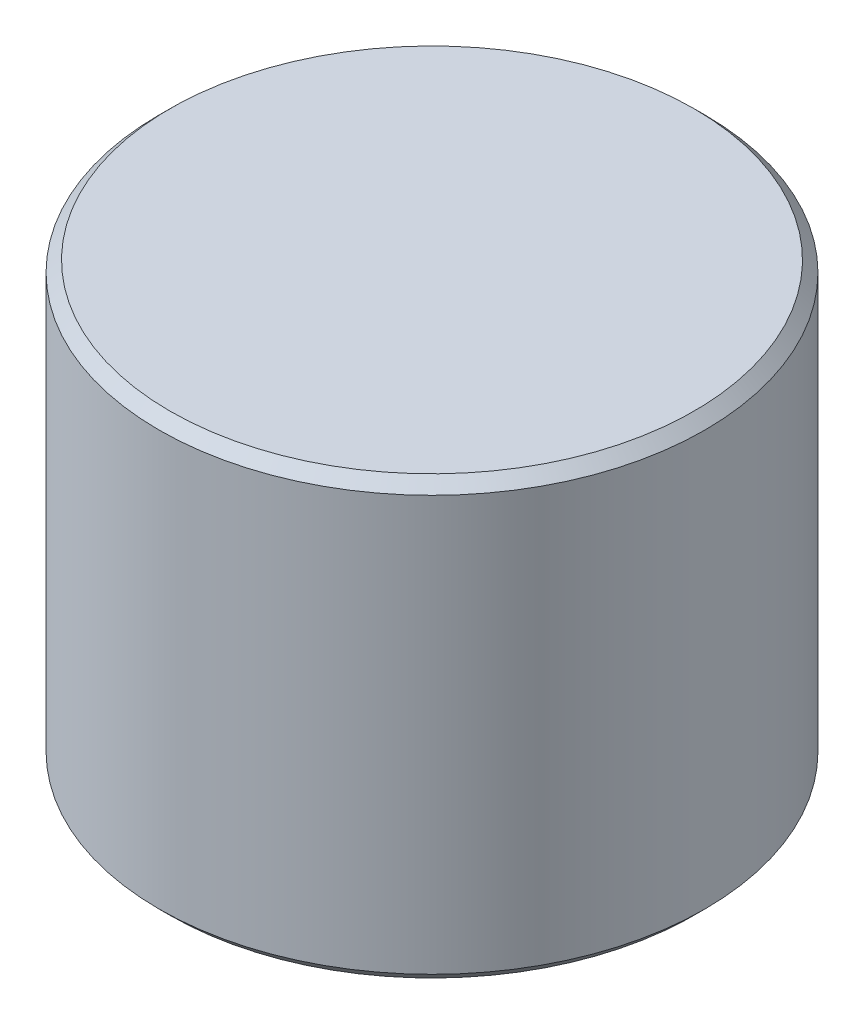
SolidWorks part; units mm, degrees
ref_plane "Front Plane" through (0, 0, 0) normal (0, 0, 1) x (1, 0, 0)
ref_plane "Top Plane" through (0, 0, 0) normal (0, 1, 0) x (1, 0, 0)
ref_plane "Right Plane" through (0, 0, 0) normal (1, 0, 0) x (0, 0, -1)
sketch "Sketch1" plane through (0, 0, 0) normal (0, 1, 0) x (1, 0, 0)
  circle A0 centre (0, 0) radius 5
  dimension "D1" = 10
extrude "Boss-Extrude1" add sketch "Sketch1" along normal blind 8
chamfer "Chamfer1" distance 0.2 angle 45 2 edges at (0, 0, 5) (0, 8, 5)
